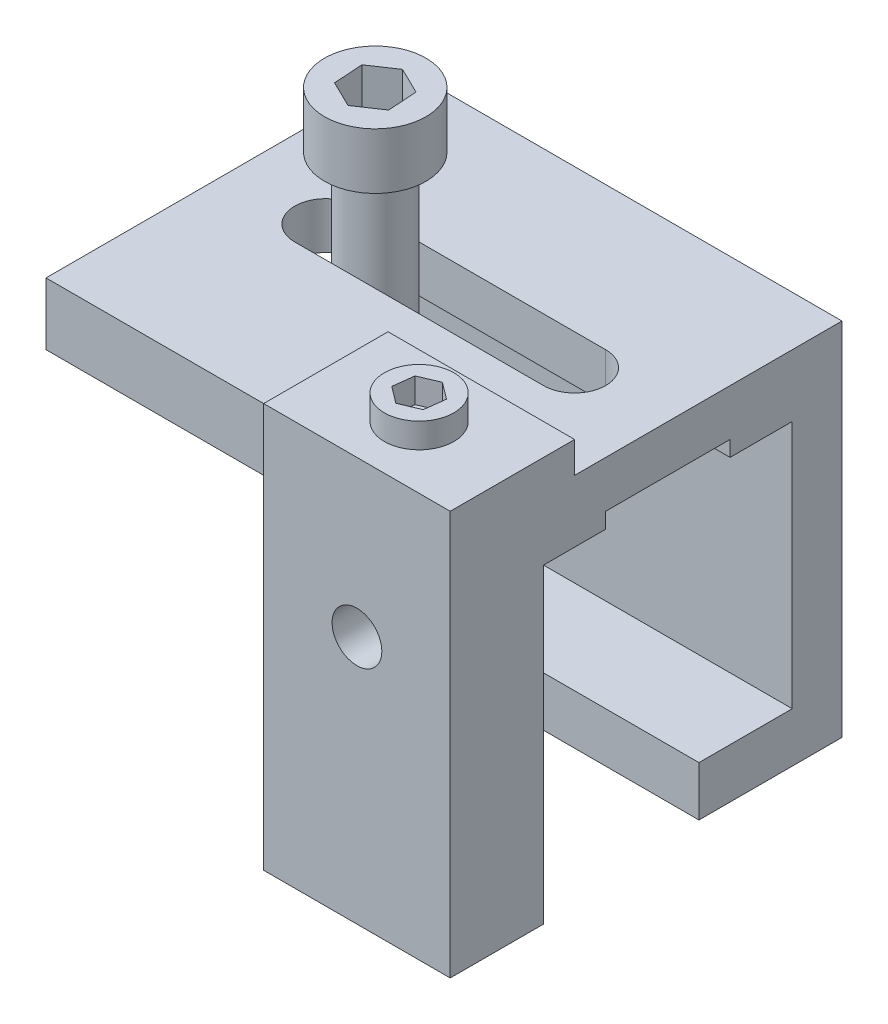
SolidWorks part; units mm, degrees
ref_plane "Front Plane" through (0, 0, 0) normal (0, 0, 1) x (1, 0, 0)
ref_plane "Top Plane" through (0, 0, 0) normal (0, 1, 0) x (1, 0, 0)
ref_plane "Right Plane" through (0, 0, 0) normal (1, 0, 0) x (0, 0, -1)
other "Configuration Table"
sketch "Sketch1" plane through (0, 0, 0) normal (0, 1, 0) x (1, 0, 0)
  line L1 (0, 0) -> (70, 0)
  line L2 (0, 0) -> (0, -50)
  line L3 (0, -50) -> (70, -50)
  line L4 (70, 0) -> (70, -50)
  dimension "D1" = 70
  dimension "D2" = 50
extrude "Boss-Extrude1" add sketch "Sketch1" along normal blind 10
sketch "Sketch2" plane through (0, 0, 0) normal (0, -1, 0) x (1, 0, 0)
  line L1 (70, 50) -> (40, 50)
  line L2 (70, 50) -> (70, 40)
  line L3 (70, 40) -> (40, 40)
  line L4 (40, 50) -> (40, 40)
  dimension "D1" = 30
  dimension "D2" = 10
extrude "Boss-Extrude2" add sketch "Sketch2" along normal blind 50
sketch "Sketch3" plane through (0, 10, 0) normal (0, 1, 0) x (1, 0, 0)
  line L1 (70, -50) -> (40, -50)
  line L2 (70, -50) -> (70, -35)
  line L3 (70, -35) -> (40, -35)
  line L4 (40, -50) -> (40, -35)
  dimension "D1" = 15
  dimension "D2" = 30
extrude "Boss-Extrude3" add sketch "Sketch3" along normal blind 5
sketch "Sketch4" plane through (0, 0, 50) normal (0, 0, 1) x (1, 0, 0)
  line L1 (40, 15) -> (70, 15)
  line L2 (40, 15) -> (40, -50)
  line L3 (40, -50) -> (70, -50)
  line L4 (70, 15) -> (70, -50)
extrude "Boss-Extrude4" add sketch "Sketch4" along normal blind 5
sketch "Sketch5" plane through (0, 10, 0) normal (0, 1, 0) x (1, 0, 0)
  line L0 (0, -20) -> (70, -20) construction
  line L1 (0, 0) -> (0, -50) construction
  line L2 (70, -35) -> (70, 0) construction
  line L3 (15, -20) -> (55, -20) construction
  line L4 (15, -15) -> (55, -15)
  line L5 (15, -25) -> (55, -25)
  line L6 (70, 0) -> (0, 0) construction
  arc A0 (15, -15) -> (15, -25) centre (15, -20) ccw
  arc A1 (55, -25) -> (55, -15) centre (55, -20) ccw
  point P8 (35, -20)
  dimension "D1" = 5
  dimension "D2" = 15
  dimension "D3" = 15
  dimension "D4" = 20
extrude "Cut-Extrude1" cut sketch "Sketch5" against normal blind 10
sketch "Sketch6" plane through (0, 0, 0) normal (-1, 0, 0) x (0, 0, 1)
  line L1 (10, 2.5) -> (30, 2.5)
  line L2 (10, 2.5) -> (10, -2.5)
  line L3 (10, -2.5) -> (30, -2.5)
  line L4 (30, 2.5) -> (30, -2.5)
  line L5 (10, 2.5) -> (30, -2.5) construction
  line L6 (10, -2.5) -> (30, 2.5) construction
  line L7 (0, 10) -> (0, 0) construction
  point P0 (20, 0)
  dimension "D1" = 20
  dimension "D2" = 5
  dimension "D3" = 20
extrude "Cut-Extrude2" cut sketch "Sketch6" against normal up to next
sketch "Sketch7" plane through (0, 15, 0) normal (0, 1, 0) x (1, 0, 0)
  line L0 (55, -55) -> (55, -35) construction
  line L1 (70, -55) -> (40, -55) construction
  line L2 (70, -35) -> (40, -35) construction
  line L4 (57.6797, -47.0222) -> (58.0911, -43.6905)
  line L5 (58.0911, -43.6905) -> (55.4115, -41.6682)
  line L6 (55.4115, -41.6682) -> (52.3203, -42.9778)
  line L7 (52.3203, -42.9778) -> (51.9089, -46.3095)
  line L8 (51.9089, -46.3095) -> (54.5885, -48.3318)
  line L9 (54.5885, -48.3318) -> (57.6797, -47.0222)
  circle A0 centre (55, -45) radius 5.5854
  circle A1 centre (55, -45) radius 2.9073 construction
extrude "Boss-Extrude5" add sketch "Sketch7" along normal blind 4
sketch "Sketch8" plane through (0, 0, 55) normal (0, 0, 1) x (1, 0, 0)
  line L0 (55, 15) -> (55, -50) construction
  line L1 (70, 15) -> (40, 15) construction
  line L2 (40, -50) -> (70, -50) construction
  circle A0 centre (55, -10) radius 4
  dimension "D2" = 8
  dimension "D1" = 25
extrude "Cut-Extrude3" cut sketch "Sketch8" against normal up to next
sketch "Sketch9" plane through (0, 0, 0) normal (0, -1, 0) x (1, 0, 0)
  line L0 (10, 20) -> (60, 20) construction
  arc A0 (15, 25) -> (15, 15) centre (15, 20) ccw construction
  arc A1 (55, 15) -> (55, 25) centre (55, 20) ccw construction
  circle A2 centre (22.9478, 20) radius 5
extrude "Boss-Extrude6" add sketch "Sketch9" along normal blind 4 and the other way blind 24 separate body
sketch "Sketch10" plane through (0, 24, 0) normal (0, 1, 0) x (1, 0, 0)
  circle A0 centre (22.9478, -20) radius 8.1588
extrude "Boss-Extrude7" add sketch "Sketch10" along normal blind 9
sketch "Sketch11" plane through (0, 33, 0) normal (0, 1, 0) x (1, 0, 0)
  line L1 (27.1834, -22.0707) -> (26.8589, -17.3672)
  line L2 (26.8589, -17.3672) -> (22.6233, -15.2965)
  line L3 (22.6233, -15.2965) -> (18.7122, -17.9293)
  line L4 (18.7122, -17.9293) -> (19.0367, -22.6328)
  line L5 (19.0367, -22.6328) -> (23.2723, -24.7035)
  line L6 (23.2723, -24.7035) -> (27.1834, -22.0707)
  circle A0 centre (22.9478, -20) radius 4.083 construction
extrude "Cut-Extrude4" cut sketch "Sketch11" against normal blind 7
sketch "Sketch12" plane through (0, 0, 0) normal (-1, 0, 0) x (0, 0, 1)
  line L0 (0, 10) -> (-8, 10)
  line L1 (-8, 10) -> (-8, -48)
  line L2 (-8, -48) -> (15, -48)
  line L3 (15, -48) -> (15, -40)
  line L4 (15, -40) -> (0, -40)
  line L5 (0, -40) -> (0, 10)
  line L6 (0, 0) -> (10, 0) construction
  dimension "D1" = 8
  dimension "D2" = 40
  dimension "D3" = 8
  dimension "D4" = 15
extrude "Boss-Extrude8" add sketch "Sketch12" against normal up to surface (70 mm away) up to face at (70, -3.75, 28.3333)
